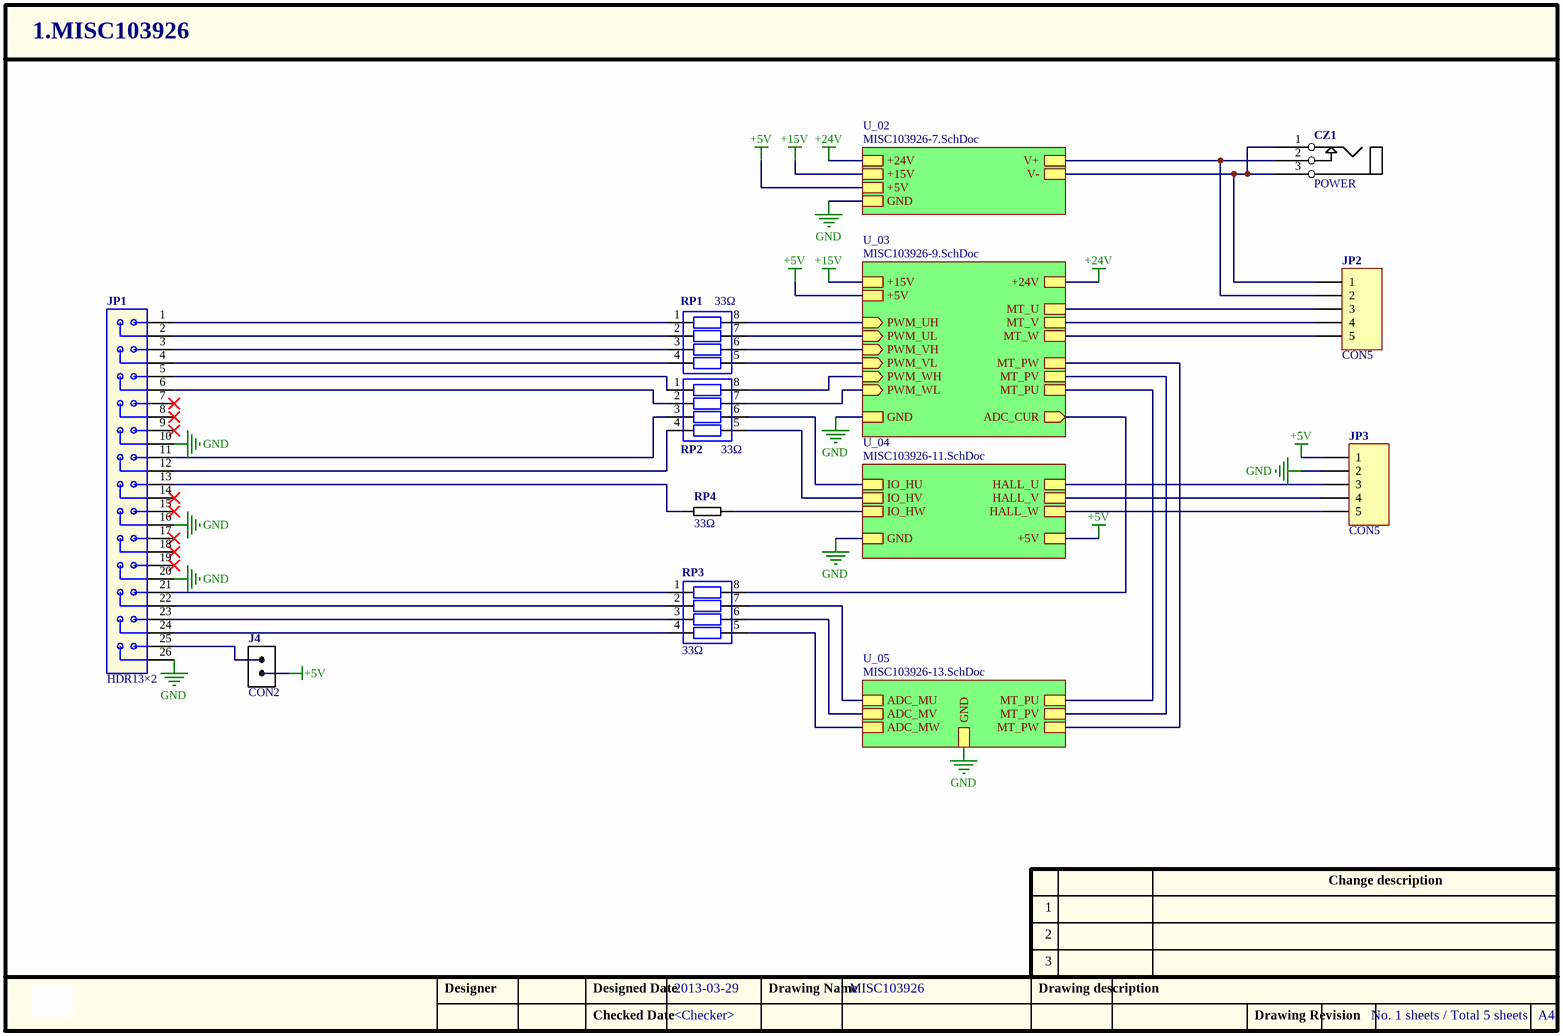
[diagram p0: MISC103926-5.SchDoc]
# Altium project MISC103926-18.PrjPCB
5 sheets, 132 parts. Net scope: hierarchical (ports join the sheet entries above them; power ports are global).
Board file: MISC103926.PcbDoc
Sheets:
  MISC103926-5.SchDoc
    U_02 = MISC103926-7.SchDoc
    U_03 = MISC103926-9.SchDoc
    U_04 = MISC103926-11.SchDoc
    U_05 = MISC103926-13.SchDoc

## Sheet MISC103926-5.SchDoc
size A4; DocumentNumber: MISC103926; SheetNumber: 1; SheetTotal: 5; DesignDate: 2013-03-29; CheckDate: <Checker>; SheetName: MISC103926

### Parts
CZ1  POWER  [POWER-AC]
J4  CON2  [SIP-2]
JP1  HDR13×2  [IDC-26]
JP2  CON5  [CON-5-5.0]
JP3  CON5  [CON-5-3.81]
RP1  33Ω  [PZ-4-0.8B]
RP2  33Ω  [PZ-4-0.8B]
RP3  33Ω  [PZ-4-0.8B]
RP4  33Ω  [0805R]

### Sub-sheets
U_02 = MISC103926-7.SchDoc: V+, V-, +24V, +15V, +5V, GND
U_03 = MISC103926-9.SchDoc: +24V, +15V, +5V, GND, ADC_CUR (out), PWM_UH (in), PWM_UL (in), PWM_VH (in), PWM_VL (in), PWM_WH (in), PWM_WL (in), MT_PU, MT_PV, MT_PW, MT_U, MT_V, MT_W
U_04 = MISC103926-11.SchDoc: IO_HU, HALL_U, IO_HV, HALL_V, IO_HW, HALL_W, +5V, GND
U_05 = MISC103926-13.SchDoc: ADC_MU, ADC_MV, ADC_MW, MT_PU, MT_PV, MT_PW, GND

### Nets
+5V: J4.1 JP3.1 ; sheet U_02/+5V, sheet U_03/+5V, sheet U_04/+5V
+15V: sheet U_02/+15V, sheet U_03/+15V
+24V: sheet U_02/+24V, sheet U_03/+24V
GND: JP1.10 JP1.16 JP1.20 JP1.26 JP3.2 ; sheet U_02/GND, sheet U_03/GND, sheet U_04/GND, sheet U_05/GND
MT_PU: sheet U_03/MT_PU, sheet U_05/MT_PU
MT_PV: sheet U_03/MT_PV, sheet U_05/MT_PV
MT_PW: sheet U_03/MT_PW, sheet U_05/MT_PW
NetC32_1: RP2.6 ; sheet U_04/IO_HU
NetC33_1: RP2.5 ; sheet U_04/IO_HV
NetC34_1: RP4.2 ; sheet U_04/IO_HW
NetC35_2: RP3.7 ; sheet U_05/ADC_MU
NetC36_2: RP3.6 ; sheet U_05/ADC_MV
NetC37_2: RP3.5 ; sheet U_05/ADC_MW
NetCZ1_1: CZ1.1(A) CZ1.3(C) JP2.1 ; sheet U_02/V-
NetCZ1_2: CZ1.2(B) JP2.2 ; sheet U_02/V+
NetJ4_2: J4.2 JP1.25
NetJP1_1: JP1.1 RP1.1
NetJP1_2: JP1.2 RP1.2
NetJP1_3: JP1.3 RP1.3
NetJP1_4: JP1.4 RP1.4
NetJP1_5: JP1.5 RP2.1
NetJP1_6: JP1.6 RP2.2
NetJP1_11: JP1.11 RP2.3
NetJP1_12: JP1.12 RP2.4
NetJP1_13: JP1.13 RP4.1
NetJP1_21: JP1.21 RP3.1
NetJP1_22: JP1.22 RP3.2
NetJP1_23: JP1.23 RP3.3
NetJP1_24: JP1.24 RP3.4
NetJP2_3: JP2.3 ; sheet U_03/MT_U
NetJP2_4: JP2.4 ; sheet U_03/MT_V
NetJP2_5: JP2.5 ; sheet U_03/MT_W
NetJP3_3: JP3.3 ; sheet U_04/HALL_U
NetJP3_4: JP3.4 ; sheet U_04/HALL_V
NetJP3_5: JP3.5 ; sheet U_04/HALL_W
NetR18_1: RP3.8 ; sheet U_03/ADC_CUR
NetRP1_5: RP1.5 ; sheet U_03/PWM_VL
NetRP1_6: RP1.6 ; sheet U_03/PWM_VH
NetRP1_7: RP1.7 ; sheet U_03/PWM_UL
NetRP1_8: RP1.8 ; sheet U_03/PWM_UH
NetRP2_7: RP2.7 ; sheet U_03/PWM_WL
NetRP2_8: RP2.8 ; sheet U_03/PWM_WH

Not connected (* = marked no-connect by the designer): JP1 7* 8* 9* 14* 15* 17* 18* 19*

### Notes on the sheet
- 1
- Change description
- 2
- 3
- Designer
- Designed Date
- Checked Date
- Drawing Name
- Drawing description
- Drawing Revision
- A4

### Library data of the parts
CZ1 = 电源座(3.5-2.1,黑色): 名称: Power socket; 型号: 3.5-2.1, black
J4 = CN-2: 名称: Shorting cap
JP1 = HDR13×2: 名称: Resistor; 封装: IDC-26
JP2 = MHDR1X5: 名称: Connector; 型号: CON-5-5.0
JP3 = MHDR1X5: Header, 5-Pin; LatestRevisionDate: 17-Jul-2002; LatestRevisionNote: Re-released for DXP Platform.; Publisher: Altium Limited
RP1-RP3 = 排阻: Resistor array; 封装: PZ-4-0.8; 型号: 33Ω×4,SMD; 名称: Resistor array
RP4 = RES(0805,33Ω): 1.01.02.0017; 名称: Resistor; 型号: 33Ω,0805

## Sheet MISC103926-7.SchDoc
size A4; DocumentNumber: MISC103926; SheetNumber: 2; SheetTotal: 5; DesignDate: 2013-03-28; CheckDate: <Checker>; SheetName: MISC103926
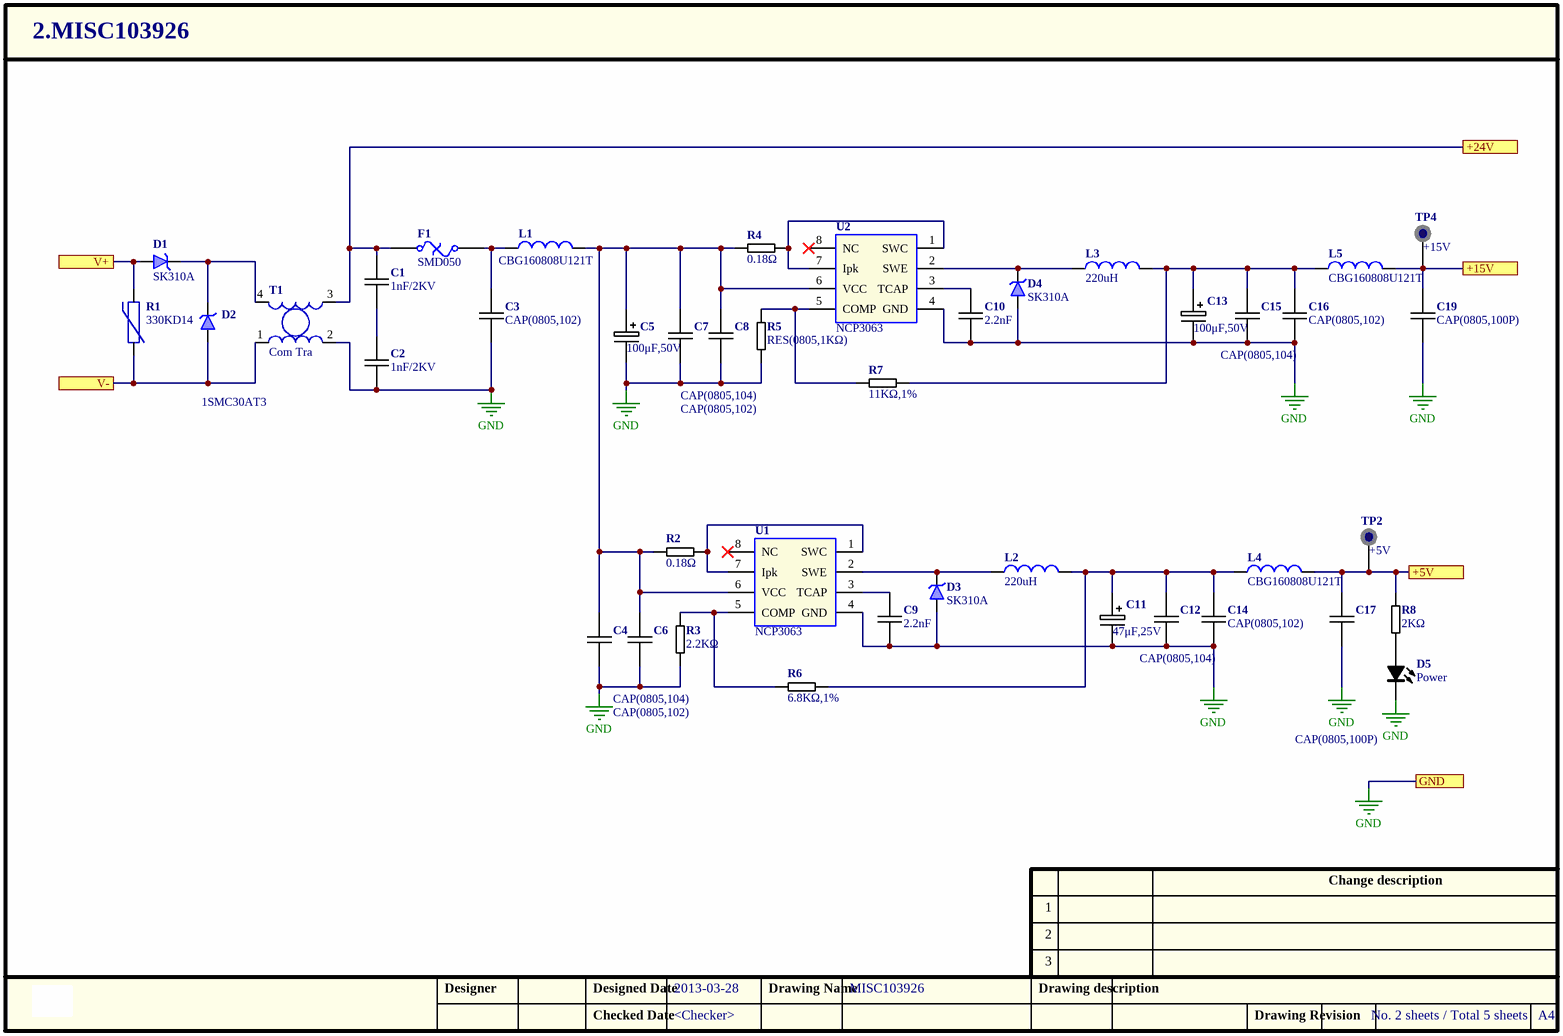
[diagram p1: MISC103926-7.SchDoc]

### Parts
C1  1nF/2KV  [1206C]
C2  1nF/2KV  [1206C]
C3  CAP(0805,102)  [0805C]
C4  CAP(0805,104)  [0805C]
C5  100μF,50V  [CAP-D]
C6  CAP(0805,102)  [0805C]
C7  CAP(0805,104)  [0805C]
C8  CAP(0805,102)  [0805C]
C9  2.2nF  [0805C]
C10  2.2nF  [0805C]
C11  47μF,25V  [CAP-D]
C12  CAP(0805,104)  [0805C]
C13  100μF,50V  [CAP-D]
C14  CAP(0805,102)  [0805C]
C15  CAP(0805,104)  [0805C]
C16  CAP(0805,102)  [0805C]
C17  CAP(0805,100P)  [0805C]
C19  CAP(0805,100P)  [0805C]
D1  SK310A  [DO-214AC]
D2  1SMC30AT3  [1SMC17AT]
D3  SK310A  [DO-214AC]
D4  SK310A  [DO-214AC]
D5  Power  [0805D]
F1  SMD050  [1812DT]
L1  CBG160808U121T  [0603C]
L2  220uH  [L-7.5S]
L3  220uH  [L-7.5S]
L4  CBG160808U121T  [0603C]
L5  CBG160808U121T  [0603C]
R1  330KD14  [AX-.3/.6]
R2  0.18Ω  [2512]
R3  2.2KΩ  [0805R]
R4  0.18Ω  [2512]
R5  RES(0805,1KΩ)  [0805R]
R6  6.8KΩ,1%  [0805R]
R7  11KΩ,1%  [0805R]
R8  2KΩ  [0805R]
T1  Com Tra  [L-2-XIAO]
TP2  +5V  [PAD(60)]
TP4  +15V  [PAD(60)]
U1  NCP3063  [SO-8]
U2  NCP3063  [SO-8]

### Ports
+5V, +15V, +24V, GND, V+, V-

### Nets
+5V: C17.1 L4.2 R8.1 TP2.1(TP) ; port +5V
+15V: C19.1 L5.2 TP4.1(TP) ; port +15V
+24V: C1.1 F1.1 T1.3 ; port +24V
GND: C2.2 C3.2 C4.2 C5.2 C6.2 C7.2 C8.2 C9.2 C10.2 C11.2 C12.2 C13.2 C14.2 C15.2 C16.2 C17.2 C19.2 D3.2 D4.2 D5.2(K) R3.2 R5.2 T1.2 U1.4(GND) U2.4(GND) ; port GND
NetC1_2: C1.2 C2.1
NetC3_1: C3.1 F1.2 L1.1
NetC4_1: C4.1 C5.1 C6.1 C7.1 C8.1 L1.2 R2.1 R4.1 U1.6(VCC) U2.6(VCC)
NetC9_1: C9.1 U1.3(TCAP)
NetC10_1: C10.1 U2.3(TCAP)
NetC11_1: C11.1 C12.1 C14.1 L2.2 L4.1 R6.2
NetC13_1: C13.1 C15.1 C16.1 L3.2 L5.1 R7.2
NetCZ1_1: D2.2 R1.2 T1.1 ; port V-
NetCZ1_2: D1.2 R1.1 ; port V+
NetD1_1: D1.1 D2.1 T1.4
NetD3_1: D3.1 L2.1 U1.2(SWE)
NetD4_1: D4.1 L3.1 U2.2(SWE)
NetD5_1: D5.1(A) R8.2
NetR2_2: R2.2 U1.1(SWC) U1.7(Ipk)
NetR3_1: R3.1 R6.1 U1.5(COMP)
NetR4_2: R4.2 U2.1(SWC) U2.7(Ipk)
NetR5_1: R5.1 R7.1 U2.5(COMP)

Not connected (* = marked no-connect by the designer): U1 8(NC)*; U2 8(NC)*

### Notes on the sheet
- 1
- Change description
- 2
- 3
- Designer
- Designed Date
- Checked Date
- Drawing Name
- Drawing description
- Drawing Revision
- A4

### Library data of the parts
C1 C2 = CAP(1206,102,2KV): 1.02.03.0003; 型号: 1nF,±10%,2KV; 封装: 1206; 名称: Capacitor
C3 C6 C8 C14 C16 = CAP(0805,102): 1.02.02.0028
C4 C7 C12 C15 = CAP(0805,104): 1.02.02.0038
C5 = CAP(电解,100UF,16V,Ф6.3×5): 名称: Tantalum capacitor; 型号: 100μF,50VD type
C9 = CAP(0805,103): 2.2nF, 24 to 5v power use; 名称: Capacitor; 封装: 0805; 型号: 222,,±10%,50V
C10 = CAP(0805,103): 2.2nF, 24 to 15 power use; 名称: Capacitor; 封装: 0805; 型号: 222,,±10%,50V
C11 = CAP(电解,100UF,16V,Ф6.3×5): 名称: Tantalum capacitor; 型号: 47μF,25V,type D
C13 = CAP(电解,100UF,16V,Ф6.3×5): SMD capacitor; 名称: Tantalum capacitor; 型号: 100μF,50V,type D
C17 C19 = CAP(0805,100P): 1.02.02.0019
D1 D3 D4 = SK310A: 名称: Diode; 型号: SK310A; 封装: DO-214AC
D2 = 1SMC30AT3: TVS diode; 名称: TVS diode; 型号: 1SMC30AT3
D5 = LED(0805,红色): 1.04.05.0001; 名称: LED; 型号: Red 0805
F1 = Fuse Thermal: Resettable fuse; 封装: 1812; 型号: SMD050; 名称: Resettable fuse
L1 L4 L5 = Inductor: 型号: CBG160808U121T,1.6×0.8×0.8mm; 封装: 0805; 名称: Ferrite bead
L2 L3 = Inductor: 型号: 220uH,Φ7.5×5mm,SMD; 名称: Inductor
R1 = 330KD14: Varistor; 名称: Varistor; 型号: 330KD14; 封装: AX-.3/.6
R2 R4 = RES(0805,0Ω): 名称: Resistor; 型号: 0.18Ω,±1%,1W; 封装: 2512
R3 = RES(0805,1KΩ): 1.01.02.0044; 名称: Resistor; 型号: 2.2K,±1%; 封装: 0805
R5 = RES(0805,1KΩ): 1.01.02.0044
R6 = RES(0805,1KΩ): 名称: Resistor; 型号: 6.8K,±1%; 封装: 0805
R7 = RES(0805,1KΩ): 名称: Resistor; 型号: 11K,±1%; 封装: 0805
R8 = RES(0805,2.2KΩ): 型号: 2K; 名称: Resistor; 封装: 0805
T1 = Com Tra: Choke coil; 型号: 0.5A-1A,15×11×16mm; 名称: Choke coil; 封装: L-2-XIAO
TP2 TP4 = 圆孔针(1P): 1.10.03.0153
U1 U2 = NCP3063: IC; 名称: IC; 封装: SO-8; 型号: NCP3063

## Sheet MISC103926-9.SchDoc
size A4; DocumentNumber: MISC103926; SheetNumber: 3; SheetTotal: 5; DesignDate: 2013-03-28; CheckDate: <Checker>; SheetName: MISC103926
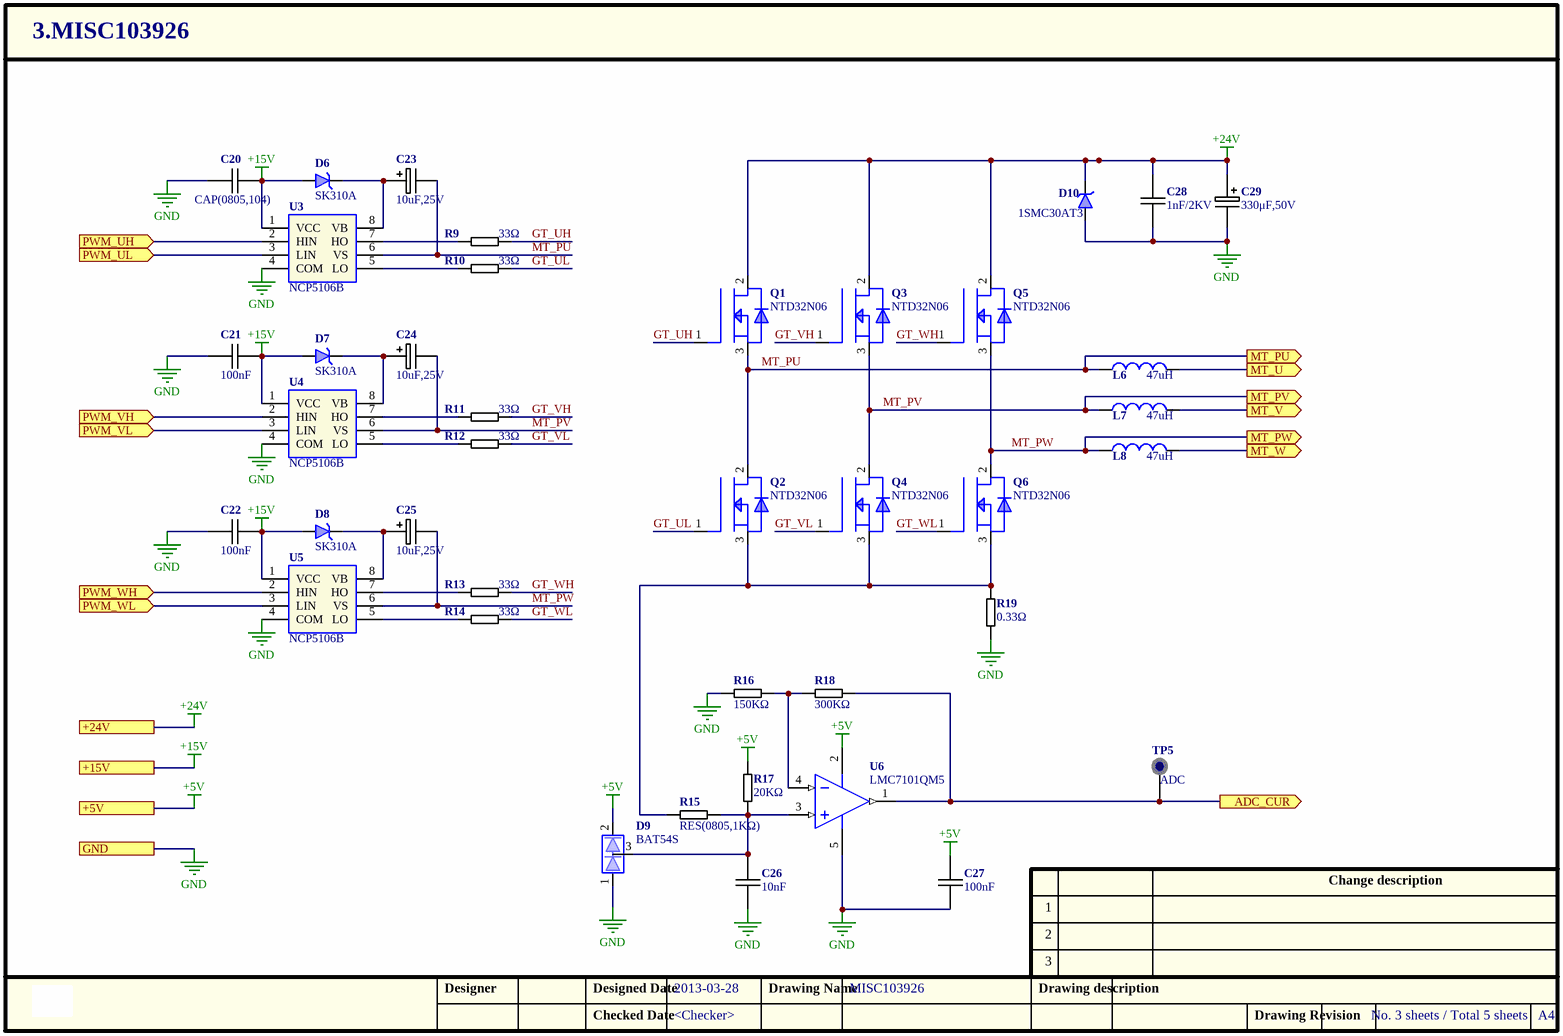
[diagram p2: MISC103926-9.SchDoc]

### Parts
C20  CAP(0805,104)  [0805C]
C21  100nF  [0805C]
C22  100nF  [0805C]
C23  10uF,25V  [CAP-C]
C24  10uF,25V  [CAP-C]
C25  10uF,25V  [CAP-C]
C26  10nF  [0805C]
C27  100nF  [0805C]
C28  1nF/2KV  [1206C]
C29  330μF,50V  [电解电容]
D6  SK310A  [DO-214AC]
D7  SK310A  [DO-214AC]
D8  SK310A  [DO-214AC]
D9  BAT54S  [SOT-23]
D10  1SMC30AT3  [1SMC17AT]
L6  47uH  [L-7.5S]
L7  47uH  [L-7.5S]
L8  47uH  [L-7.5S]
Q1  NTD32N06  [DPAK-3]
Q2  NTD32N06  [DPAK-3]
Q3  NTD32N06  [DPAK-3]
Q4  NTD32N06  [DPAK-3]
Q5  NTD32N06  [DPAK-3]
Q6  NTD32N06  [DPAK-3]
R9  33Ω  [0805R]
R10  33Ω  [0805R]
R11  33Ω  [0805R]
R12  33Ω  [0805R]
R13  33Ω  [0805R]
R14  33Ω  [0805R]
R15  RES(0805,1KΩ)  [0805R]
R16  150KΩ  [0805R]
R17  20KΩ  [0805R]
R18  300KΩ  [0805R]
R19  0.33Ω  [2512]
TP5  ADC  [PAD(60)]
U3  NCP5106B  [SO-8]
U4  NCP5106B  [SO-8]
U5  NCP5106B  [SO-8]
U6  LMC7101QM5  [MF05A_N]

### Ports
+5V, +15V, +24V, ADC_CUR (out), GND, MT_PU, MT_PV, MT_PW, MT_U, MT_V, MT_W, PWM_UH (in), PWM_UL (in), PWM_VH (in), PWM_VL (in), PWM_WH (in), PWM_WL (in)

### Nets
+5V: C27.2 D9.2 R17.1 U6.2(V+) ; port +5V
+15V: C20.2 C21.2 C22.2 D6.2 D7.2 D8.2 U3.1(VCC) U4.1(VCC) U5.1(VCC) ; port +15V
+24V: C28.1 C29.1 D10.1 Q1.2 Q3.2 Q5.2 ; port +24V
GND: C20.1 C21.1 C22.1 C26.1 C27.1 C28.2 C29.2 D9.1 D10.2 R16.2 R19.1 U3.4(COM) U4.4(COM) U5.4(COM) U6.5(V-) ; port GND
GT_UH: Q1.1 R9.2
GT_UL: Q2.1 R10.2
GT_VH: Q3.1 R11.2
GT_VL: Q4.1 R12.2
GT_WH: Q5.1 R13.2
GT_WL: Q6.1 R14.2
MT_PU: C23.2 L6.1 Q1.3 Q2.2 U3.6(VS) ; port MT_PU
MT_PV: C24.2 L7.1 Q3.3 Q4.2 U4.6(VS) ; port MT_PV
MT_PW: C25.2 L8.1 Q5.3 Q6.2 U5.6(VS) ; port MT_PW
NetC23_1: C23.1 D6.1 U3.8(VB)
NetC24_1: C24.1 D7.1 U4.8(VB)
NetC25_1: C25.1 D8.1 U5.8(VB)
NetC26_2: C26.2 D9.3 R15.2 R17.2 U6.3(IN+)
NetJP2_3: L6.2 ; port MT_U
NetJP2_4: L7.2 ; port MT_V
NetJP2_5: L8.2 ; port MT_W
NetQ2_3: Q2.3 Q4.3 Q6.3 R15.1 R19.2
NetR9_1: R9.1 U3.7(HO)
NetR10_1: R10.1 U3.5(LO)
NetR11_1: R11.1 U4.7(HO)
NetR12_1: R12.1 U4.5(LO)
NetR13_1: R13.1 U5.7(HO)
NetR14_1: R14.1 U5.5(LO)
NetR16_1: R16.1 R18.2 U6.4(IN-)
NetR18_1: R18.1 TP5.1(TP) U6.1(OUT) ; port ADC_CUR
NetRP1_5: U4.3(LIN) ; port PWM_VL
NetRP1_6: U4.2(HIN) ; port PWM_VH
NetRP1_7: U3.3(LIN) ; port PWM_UL
NetRP1_8: U3.2(HIN) ; port PWM_UH
NetRP2_7: U5.3(LIN) ; port PWM_WL
NetRP2_8: U5.2(HIN) ; port PWM_WH

### Notes on the sheet
- 1
- Change description
- 2
- 3
- Designer
- Designed Date
- Checked Date
- Drawing Name
- Drawing description
- Drawing Revision
- A4

### Library data of the parts
C20 = CAP(0805,104): 1.02.02.0038
C21 C22 C27 = CAP(0805,104): 1.02.02.0038; 名称: Capacitor; 型号: 0805,104
C23 = CAP(电解,10UF,25V,Ф4×7): SMD capacitor; 名称: Tantalum capacitor; 型号: 10uF,25V,type C
C24 C25 = CAP(电解,10UF,25V,Ф4×7): 名称: Tantalum capacitor; 型号: 10uF,25V,type C
C26 = CAP(0805,103): 1.02.02.0032; 名称: Capacitor; 型号: 103,0805
C28 = CAP(1206,102,2KV): as C1 on sheet MISC103926-7
C29 = CAP(电解,100UF,16V,Ф6.3×5): Electrolytic capacitor; 型号: Capacitor,330μF,50V,Ф10×16; 名称: Electrolytic capacitor
D6-D8 = SK310A: 名称: Diode; 型号: SK310A; 封装: DO-214AC
D9 = BAT54S: Diode; 名称: Diode; 型号: BAT54S
D10 = 1SMC30AT3: TVS diode; 名称: TVS diode; 型号: 1SMC30AT3
L6-L8 = Inductor: 型号: 47uH,1A,Φ7.5×5mm,SMD; 名称: Inductor
Q1-Q6 = NTD32N06: MOSFET; 封装: DPAK; 名称: MOSFET; 型号: NTD32N06
R9-R14 = RES(0805,33Ω): 1.01.02.0017; 名称: Resistor; 型号: 33Ω,0805
R15 = RES(0805,1KΩ): 1.01.02.0044
R16 = RES(0805,300KΩ): 名称: Resistor; 型号: 150KΩ,0805
R17 = RES(0805,300KΩ): 名称: Resistor; 型号: 20KΩ,0805
R18 = RES(0805,300KΩ): 1.01.02.0097; 名称: Resistor; 型号: 300KΩ,0805
R19 = RES(0805,0Ω): 1.01.02.0001; 名称: Resistor; 型号: 0.33Ω,±1%,1W; 封装: 2512
TP5 = 圆孔针(1P): 1.10.03.0153
U3-U5 = NCP5106B: IC; 名称: IC; 封装: SO-8; 型号: NCP5106B
U6 = LMC7101QM5: Tiny Low Power Operational Amplifier with Rail-to-Rail Input and Output; Manufacturer: National Semiconductor; CompType: Amplifiers; PackageTopMarking: AT6A*XTT; PowerWise: N; Published: 9-Oct-2009; DatasheetVersion: Jun-2009; PackageVersion: revD, Aug-2008; PackageReference: MF05A; PackageDescription: Molded SOT-23, .115 x .063 x .040 in Body, 5 Lead, .0375 in Pitch; PartNumber: LMC7101QM5; RoHS: Y; PinCount: 5; ComponentLink1Description: LMC7101 Datasheet; ComponentLink1URL: http://example.com/ds/LM/LMC7101.pdf; ComponentLink2Description: LMC7101 Web Page; ComponentLink3Description: MF05A Package Page; Publisher: Altium Limited

## Sheet MISC103926-11.SchDoc
size A4; DocumentNumber: MISC103926; SheetNumber: 4; SheetTotal: 5; DesignDate: 2013-03-29; CheckDate: <Checker>; SheetName: MISC103926
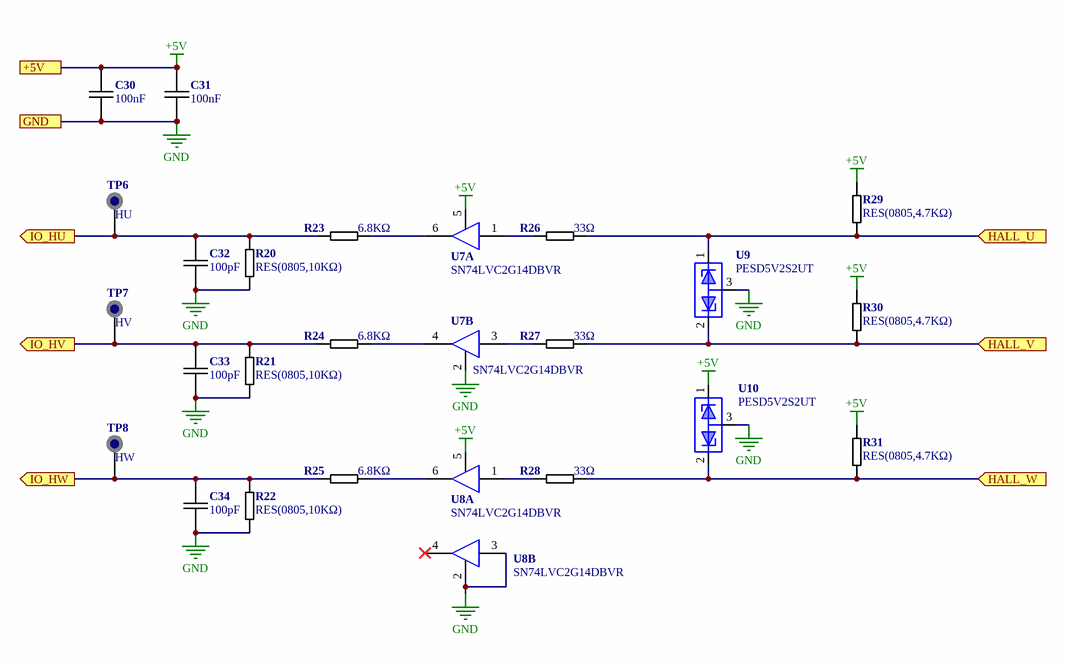
[diagram p3: MISC103926-11.SchDoc]

### Parts
C30  100nF  [0805C]
C31  100nF  [0805C]
C32  100pF  [0805C]
C33  100pF  [0805C]
C34  100pF  [0805C]
R20  RES(0805,10KΩ)  [0805R]
R21  RES(0805,10KΩ)  [0805R]
R22  RES(0805,10KΩ)  [0805R]
R23  6.8KΩ  [0805R]
R24  6.8KΩ  [0805R]
R25  6.8KΩ  [0805R]
R26  33Ω  [0805R]
R27  33Ω  [0805R]
R28  33Ω  [0805R]
R29  RES(0805,4.7KΩ)  [0805R]
R30  RES(0805,4.7KΩ)  [0805R]
R31  RES(0805,4.7KΩ)  [0805R]
TP6  HU  [PAD(60)]
TP7  HV  [PAD(60)]
TP8  HW  [PAD(60)]
U7  SN74LVC2G14DBVR  [SOT-23-6]  (parts A,B of 2)
U8  SN74LVC2G14DBVR  [SOT-23-6]  (parts A,B of 2)
U9  PESD5V2S2UT  [SOT-23]
U10  PESD5V2S2UT  [SOT-23]

### Ports
+5V, GND, HALL_U, HALL_V, HALL_W, IO_HU, IO_HV, IO_HW

### Nets
+5V: C30.1 C31.2 R29.1 R30.1 R31.1 U7.5 U8.5 U10.1 ; port +5V
GND: C30.2 C31.1 C32.2 C33.2 C34.2 R20.2 R21.2 R22.2 U7.2 U8.2 U8.3 U9.3 U10.3 ; port GND
NetC32_1: C32.1 R20.1 R23.1 TP6.1(TP) ; port IO_HU
NetC33_1: C33.1 R21.1 R24.1 TP7.1(TP) ; port IO_HV
NetC34_1: C34.1 R22.1 R25.1 TP8.1(TP) ; port IO_HW
NetJP3_3: R26.2 R29.2 U9.1 ; port HALL_U
NetJP3_4: R27.2 R30.2 U9.2 ; port HALL_V
NetJP3_5: R28.2 R31.2 U10.2 ; port HALL_W
NetR23_2: R23.2 U7.6
NetR24_2: R24.2 U7.4
NetR25_2: R25.2 U8.6
NetR26_1: R26.1 U7.1
NetR27_1: R27.1 U7.3
NetR28_1: R28.1 U8.1

Not connected (* = marked no-connect by the designer): U8 4*

### Notes on the sheet
- 1
- Change description
- 2
- 3
- Designer
- Designed Date
- Checked Date
- Drawing Name
- Drawing description
- Drawing Revision
- A4

### Library data of the parts
C30 C31 = CAP(0805,104): 1.02.02.0038; 名称: Capacitor; 型号: 0805,104
C32-C34 = CAP(0805,100P): 1.02.02.0019; 名称: Capacitor; 型号: 100pF,±5%,50V; 封装: 0805
R20-R22 = RES(0805,10KΩ): 1.01.02.0067
R23-R25 = RES(0805,33Ω): 名称: Resistor; 型号: 6.8KΩ,0805
R26-R28 = RES(0805,33Ω): 1.01.02.0017; 名称: Resistor; 型号: 33Ω,0805
R29-R31 = RES(0805,4.7KΩ): 1.01.02.0059
TP6-TP8 = 圆孔针(1P): 1.10.03.0153
U7 U8 = SN74LVC2G14DBVR: IC; 封装: SOT-23-6L; 名称: IC; 型号: SN74LVC2G14DBVR
U9 U10 = PESD5V2S2UT: IC; 名称: IC; 封装: SOT-23; 型号: PESD5V2S2UT

## Sheet MISC103926-13.SchDoc
size A4; DocumentNumber: MISC103926; SheetNumber: 5; SheetTotal: 5; DesignDate: 2013-03-29; CheckDate: <Checker>; SheetName: MISC103926
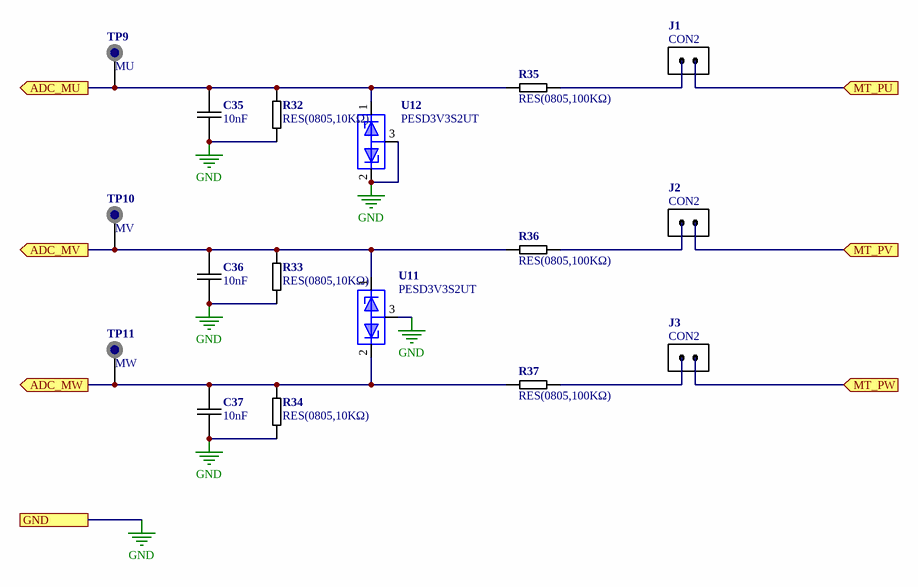
[diagram p4: MISC103926-13.SchDoc]

### Parts
C35  10nF  [0805C]
C36  10nF  [0805C]
C37  10nF  [0805C]
J1  CON2  [SIP-2]
J2  CON2  [SIP-2]
J3  CON2  [SIP-2]
R32  RES(0805,10KΩ)  [0805R]
R33  RES(0805,10KΩ)  [0805R]
R34  RES(0805,10KΩ)  [0805R]
R35  RES(0805,100KΩ)  [0805R]
R36  RES(0805,100KΩ)  [0805R]
R37  RES(0805,100KΩ)  [0805R]
TP9  MU  [PAD(60)]
TP10  MV  [PAD(60)]
TP11  MW  [PAD(60)]
U11  PESD3V3S2UT  [SOT-23]
U12  PESD3V3S2UT  [SOT-23]

### Ports
ADC_MU, ADC_MV, ADC_MW, GND, MT_PU, MT_PV, MT_PW

### Nets
GND: C35.1 C36.1 C37.1 R32.2 R33.2 R34.2 U11.3 U12.2 U12.3 ; port GND
MT_PU: J1.2 ; port MT_PU
MT_PV: J2.2 ; port MT_PV
MT_PW: J3.2 ; port MT_PW
NetC35_2: C35.2 R32.1 R35.1 TP9.1(TP) U12.1 ; port ADC_MU
NetC36_2: C36.2 R33.1 R36.1 TP10.1(TP) U11.1 ; port ADC_MV
NetC37_2: C37.2 R34.1 R37.1 TP11.1(TP) U11.2 ; port ADC_MW
NetJ1_1: J1.1 R35.2
NetJ2_1: J2.1 R36.2
NetJ3_1: J3.1 R37.2

### Notes on the sheet
- 1
- Change description
- 2
- 3
- Designer
- Designed Date
- Checked Date
- Drawing Name
- Drawing description
- Drawing Revision
- A4

### Library data of the parts
C35-C37 = CAP(0805,103): as C26 on sheet MISC103926-9
J1-J3 = CN-2: 名称: Shorting cap
R32-R34 = RES(0805,10KΩ): 1.01.02.0067
R35-R37 = RES(0805,100KΩ): 1.01.02.0092
TP9-TP11 = 圆孔针(1P): 1.10.03.0153
U11 U12 = PESD3V3S2UT: IC; 名称: IC; 封装: SOT-23; 型号: PESD3V3S2UT

## Nets that join several sheets
+5V: MISC103926-5 (J4.1 JP3.1), MISC103926-7 (C17.1 L4.2 R8.1 TP2.1), MISC103926-9 (C27.2 D9.2 R17.1 U6.2), MISC103926-11 (8 pins)
+15V: MISC103926-7 (C19.1 L5.2 TP4.1), MISC103926-9 (9 pins)
+24V: MISC103926-7 (C1.1 F1.1 T1.3), MISC103926-9 (6 pins)
GND: MISC103926-5 (5 pins), MISC103926-7 (25 pins), MISC103926-9 (15 pins), MISC103926-11 (13 pins), MISC103926-13 (9 pins)
MT_PU: MISC103926-9 (5 pins), MISC103926-13 (J1.2)
MT_PV: MISC103926-9 (5 pins), MISC103926-13 (J2.2)
MT_PW: MISC103926-9 (5 pins), MISC103926-13 (J3.2)
NetC32_1: MISC103926-5 (RP2.6), MISC103926-11 (C32.1 R20.1 R23.1 TP6.1)
NetC33_1: MISC103926-5 (RP2.5), MISC103926-11 (C33.1 R21.1 R24.1 TP7.1)
NetC34_1: MISC103926-5 (RP4.2), MISC103926-11 (C34.1 R22.1 R25.1 TP8.1)
NetC35_2: MISC103926-5 (RP3.7), MISC103926-13 (5 pins)
NetC36_2: MISC103926-5 (RP3.6), MISC103926-13 (5 pins)
NetC37_2: MISC103926-5 (RP3.5), MISC103926-13 (5 pins)
NetCZ1_1: MISC103926-5 (CZ1.1 CZ1.3 JP2.1), MISC103926-7 (D2.2 R1.2 T1.1)
NetCZ1_2: MISC103926-5 (CZ1.2 JP2.2), MISC103926-7 (D1.2 R1.1)
NetJP2_3: MISC103926-5 (JP2.3), MISC103926-9 (L6.2)
NetJP2_4: MISC103926-5 (JP2.4), MISC103926-9 (L7.2)
NetJP2_5: MISC103926-5 (JP2.5), MISC103926-9 (L8.2)
NetJP3_3: MISC103926-5 (JP3.3), MISC103926-11 (R26.2 R29.2 U9.1)
NetJP3_4: MISC103926-5 (JP3.4), MISC103926-11 (R27.2 R30.2 U9.2)
NetJP3_5: MISC103926-5 (JP3.5), MISC103926-11 (R28.2 R31.2 U10.2)
NetR18_1: MISC103926-5 (RP3.8), MISC103926-9 (R18.1 TP5.1 U6.1)
NetRP1_5: MISC103926-5 (RP1.5), MISC103926-9 (U4.3)
NetRP1_6: MISC103926-5 (RP1.6), MISC103926-9 (U4.2)
NetRP1_7: MISC103926-5 (RP1.7), MISC103926-9 (U3.3)
NetRP1_8: MISC103926-5 (RP1.8), MISC103926-9 (U3.2)
NetRP2_7: MISC103926-5 (RP2.7), MISC103926-9 (U5.3)
NetRP2_8: MISC103926-5 (RP2.8), MISC103926-9 (U5.2)